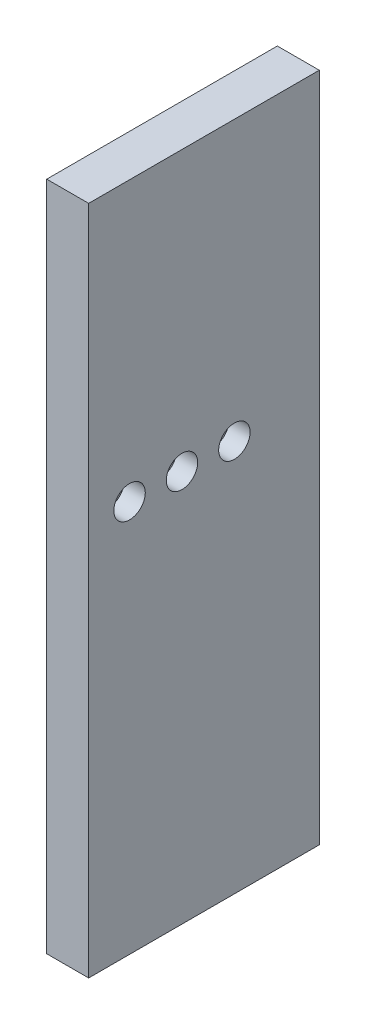
from build123d import *

# Parameters (mm, degrees)
SKETCH1_W                                = 20
SKETCH1_H                                = 320
BOSS_EXTRUDE1_DEPTH                      = 110
CBORE_FOR_M10_HEX_HEAD_BOLT1_D           = 11
CBORE_FOR_M10_HEX_HEAD_BOLT1_DEPTH       = 22.25
CBORE_FOR_M10_HEX_HEAD_BOLT1_CBORE_D     = 15
CBORE_FOR_M10_HEX_HEAD_BOLT1_CBORE_DEPTH = 10
CBORE_FOR_M10_HEX_HEAD_BOLT1_TIP         = 3.304733405


with BuildPart() as part:
    # Sketch1 → Boss-Extrude1 (new body)
    with BuildSketch(Plane.XY):
        with Locations((110, 300)):
            Rectangle(SKETCH1_W, SKETCH1_H)
    extrude(amount=BOSS_EXTRUDE1_DEPTH)

    # CBORE for M10 Hex Head Bolt1
    with Locations(Plane(origin=(120, 0, 0), x_dir=(0, 0, -1), z_dir=(1, 0, 0))):
        with Locations((-90.49, 327), (-65.49, 327), (-40.49, 327)):
            CounterBoreHole(CBORE_FOR_M10_HEX_HEAD_BOLT1_D / 2, CBORE_FOR_M10_HEX_HEAD_BOLT1_CBORE_D / 2, CBORE_FOR_M10_HEX_HEAD_BOLT1_CBORE_DEPTH, depth=CBORE_FOR_M10_HEX_HEAD_BOLT1_DEPTH)
            with Locations((0, 0, -(CBORE_FOR_M10_HEX_HEAD_BOLT1_DEPTH + CBORE_FOR_M10_HEX_HEAD_BOLT1_TIP / 2))):  # 118° drill point
                Cone(0, CBORE_FOR_M10_HEX_HEAD_BOLT1_D / 2, CBORE_FOR_M10_HEX_HEAD_BOLT1_TIP, mode=Mode.SUBTRACT)


solid = part.part
